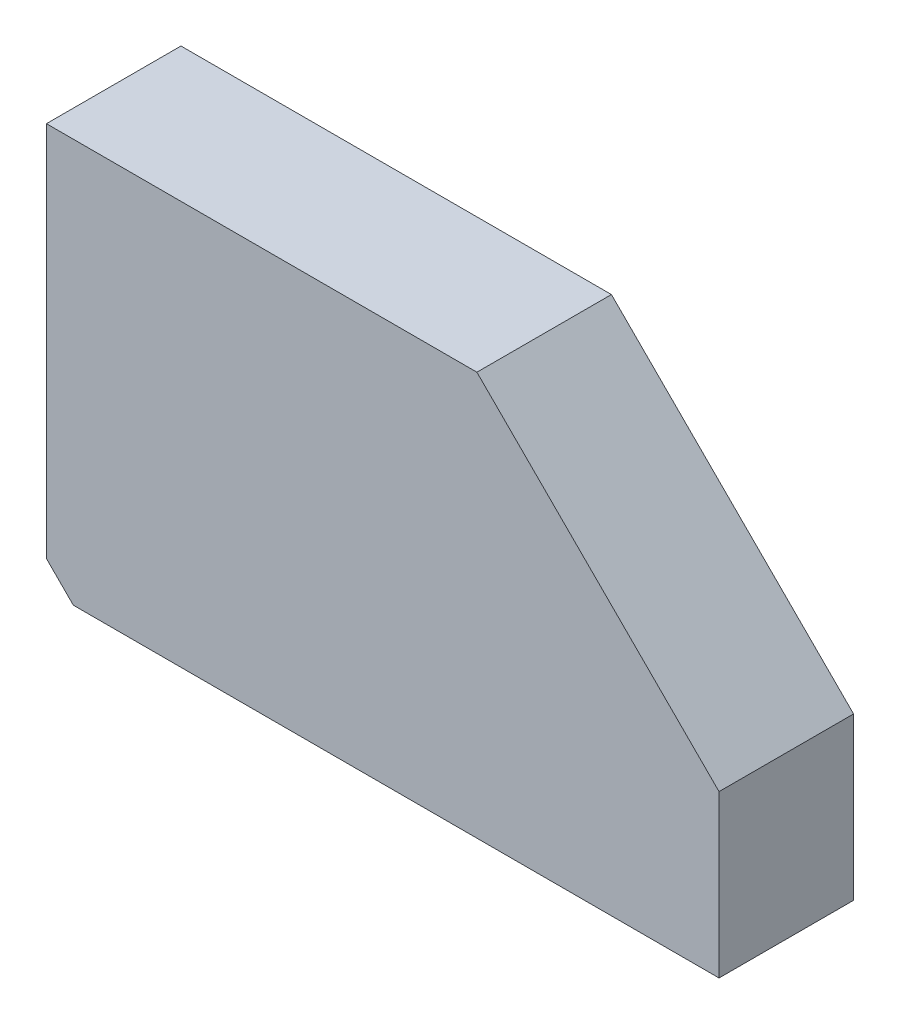
from build123d import *

# Parameters (mm, degrees)
EXTRUDE_1_DEPTH        = 10
CHAMFER_1_SIZE         = 2
HOLE_WIZARD_M5_1_D     = 4.2
HOLE_WIZARD_M5_1_DEPTH = 14
HOLE_WIZARD_M5_1_TIP   = 1.2618073
HOLE_WIZARD_M5_2_D     = 4.2
HOLE_WIZARD_M5_2_DEPTH = 14
HOLE_WIZARD_M5_2_TIP   = 1.2618073


with BuildPart() as part:
    # 草图1 → 凸台-拉伸1 (new body)
    with BuildSketch(Plane.XY):
        Polygon((62, -20.911504847), (12, -20.911504847), (12, 9.088495153), (44, 9.088495153), (62, -8.911504847), align=None)
    extrude(amount=EXTRUDE_1_DEPTH)

    # 倒角1
    chamfer_1_edges = [part.edges().sort_by_distance(p)[0] for p in [
        (12, -20.911504847, 5),
    ]]
    chamfer(chamfer_1_edges, length=CHAMFER_1_SIZE)

    # M5 螺纹孔1
    with Locations(Plane.ZY.offset(-12)):
        with Locations((5, -10.911504847), (5, 1.088495153)):
            Hole(HOLE_WIZARD_M5_1_D / 2, depth=HOLE_WIZARD_M5_1_DEPTH)
            with Locations((0, 0, -(HOLE_WIZARD_M5_1_DEPTH + HOLE_WIZARD_M5_1_TIP / 2))):  # 118° drill point
                Cone(0, HOLE_WIZARD_M5_1_D / 2, HOLE_WIZARD_M5_1_TIP, mode=Mode.SUBTRACT)

    # M5 螺纹孔2
    with Locations(Plane(origin=(0, -20.911504847, 0), x_dir=(-1, 0, 0), z_dir=(0, -1, 0))):
        with Locations((-30, -5), (-50, -5)):
            Hole(HOLE_WIZARD_M5_2_D / 2, depth=HOLE_WIZARD_M5_2_DEPTH)
            with Locations((0, 0, -(HOLE_WIZARD_M5_2_DEPTH + HOLE_WIZARD_M5_2_TIP / 2))):  # 118° drill point
                Cone(0, HOLE_WIZARD_M5_2_D / 2, HOLE_WIZARD_M5_2_TIP, mode=Mode.SUBTRACT)


solid = part.part
